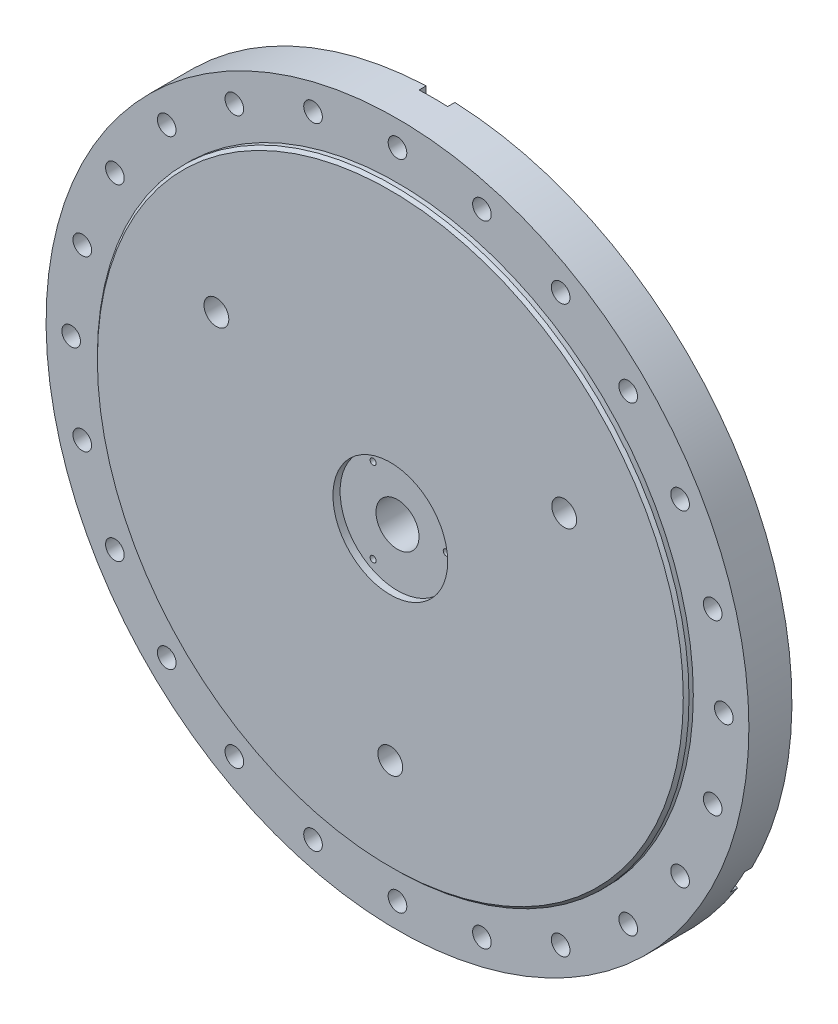
SolidWorks part; units mm, degrees
ref_plane "Front Plane" through (0, 0, 0) normal (0, 0, 1) x (1, 0, 0)
ref_plane "Top Plane" through (0, 0, 0) normal (0, 1, 0) x (1, 0, 0)
ref_plane "Right Plane" through (0, 0, 0) normal (1, 0, 0) x (0, 0, -1)
sketch "Sketch1" plane through (0, 0, 0) normal (0, 0, 1) x (1, 0, 0)
  circle A50 centre (114.9929, 70) radius 8.647 construction
  circle A51 centre (97.4929, 100.3109) radius 1.621 construction
  circle A52 centre (132.4929, 39.6891) radius 1.621 construction
  circle A53 centre (13.7494, 235) radius 2.067 construction
  circle A54 centre (207.2653, -100.1795) radius 2.067 construction
  circle A55 centre (214.9531, -72.8638) radius 2.4585 construction
  circle A56 centre (201.0967, -64.8638) radius 2.4585 construction
  circle A57 centre (187.2403, -56.8638) radius 2.4585 construction
  circle A58 centre (173.3839, -48.8638) radius 2.4585 construction
  circle A59 centre (159.5275, -40.8638) radius 2.4585 construction
  circle A60 centre (145.6711, -32.8638) radius 2.4585 construction
  circle A61 centre (131.8147, -24.8638) radius 2.4585 construction
  circle A62 centre (117.9583, -16.8638) radius 2.4585 construction
  circle A63 centre (104.1019, -8.8638) radius 2.4585 construction
  circle A64 centre (90.2455, -0.8638) radius 2.4585 construction
  circle A65 centre (76.3891, 7.1362) radius 2.4585 construction
  circle A66 centre (62.5327, 15.1362) radius 2.4585 construction
  circle A67 centre (48.6763, 23.1362) radius 2.4585 construction
  circle A68 centre (34.8199, 31.1362) radius 2.4585 construction
  circle A69 centre (41.2494, 228) radius 2.4585 construction
  circle A70 centre (41.2494, 212) radius 2.4585 construction
  circle A71 centre (41.2494, 196) radius 2.4585 construction
  circle A72 centre (41.2494, 180) radius 2.4585 construction
  circle A73 centre (41.2494, 164) radius 2.4585 construction
  circle A74 centre (41.2494, 148) radius 2.4585 construction
  circle A75 centre (41.2494, 132) radius 2.4585 construction
  circle A76 centre (41.2494, 116) radius 2.4585 construction
  circle A77 centre (41.2494, 100) radius 2.4585 construction
  circle A78 centre (41.2494, 84) radius 2.4585 construction
  circle A79 centre (41.2494, 68) radius 2.4585 construction
  circle A80 centre (41.2494, 52) radius 2.4585 construction
  circle A81 centre (41.2494, 36) radius 2.4585 construction
  circle A82 centre (41.2494, 20) radius 2.4585 construction
  circle A83 centre (-127.4942, 70) radius 8.647 construction
  circle A84 centre (-144.9942, 39.6891) radius 1.621 construction
  circle A85 centre (-109.9942, 100.3109) radius 1.621 construction
  circle A86 centre (-219.7666, -100.1795) radius 2.067 construction
  circle A87 centre (-26.2506, 235) radius 2.067 construction
  circle A88 centre (-227.4544, -72.8638) radius 2.4585 construction
  circle A89 centre (-213.598, -64.8638) radius 2.4585 construction
  circle A90 centre (-199.7416, -56.8638) radius 2.4585 construction
  circle A91 centre (-185.8852, -48.8638) radius 2.4585 construction
  circle A92 centre (-172.0288, -40.8638) radius 2.4585 construction
  circle A93 centre (-158.1724, -32.8638) radius 2.4585 construction
  circle A94 centre (-144.316, -24.8638) radius 2.4585 construction
  circle A95 centre (-130.4596, -16.8638) radius 2.4585 construction
  circle A96 centre (-116.6032, -8.8638) radius 2.4585 construction
  circle A97 centre (-102.7468, -0.8638) radius 2.4585 construction
  circle A98 centre (-88.8904, 7.1362) radius 2.4585 construction
  circle A99 centre (-75.034, 15.1362) radius 2.4585 construction
  circle A100 centre (-61.1776, 23.1362) radius 2.4585 construction
  circle A101 centre (-47.3212, 31.1362) radius 2.4585 construction
  circle A102 centre (-53.7506, 228) radius 2.4585 construction
  circle A103 centre (-53.7506, 212) radius 2.4585 construction
  circle A104 centre (-53.7506, 196) radius 2.4585 construction
  circle A105 centre (-53.7506, 180) radius 2.4585 construction
  circle A106 centre (-53.7506, 164) radius 2.4585 construction
  circle A107 centre (-53.7506, 148) radius 2.4585 construction
  circle A108 centre (-53.7506, 132) radius 2.4585 construction
  circle A109 centre (-53.7506, 116) radius 2.4585 construction
  circle A110 centre (-53.7506, 100) radius 2.4585 construction
  circle A111 centre (-53.7506, 84) radius 2.4585 construction
  circle A112 centre (-53.7506, 68) radius 2.4585 construction
  circle A113 centre (-53.7506, 52) radius 2.4585 construction
  circle A114 centre (-53.7506, 36) radius 2.4585 construction
  circle A115 centre (-53.7506, 20) radius 2.4585 construction
  circle A116 centre (-6.2506, -140) radius 8.647 construction
  circle A117 centre (28.7494, -140) radius 1.621 construction
  circle A118 centre (-41.2506, -140) radius 1.621 construction
  circle A119 centre (-199.7666, -134.8205) radius 2.067 construction
  circle A120 centre (187.2653, -134.8205) radius 2.067 construction
  circle A121 centre (167.4531, -155.1362) radius 2.4585 construction
  circle A122 centre (153.5967, -147.1362) radius 2.4585 construction
  circle A123 centre (139.7403, -139.1362) radius 2.4585 construction
  circle A124 centre (125.8839, -131.1362) radius 2.4585 construction
  circle A125 centre (112.0275, -123.1362) radius 2.4585 construction
  circle A126 centre (98.1711, -115.1362) radius 2.4585 construction
  circle A127 centre (84.3147, -107.1362) radius 2.4585 construction
  circle A128 centre (70.4583, -99.1362) radius 2.4585 construction
  circle A129 centre (56.6019, -91.1362) radius 2.4585 construction
  circle A130 centre (42.7455, -83.1362) radius 2.4585 construction
  circle A131 centre (28.8891, -75.1362) radius 2.4585 construction
  circle A132 centre (15.0327, -67.1362) radius 2.4585 construction
  circle A133 centre (1.1763, -59.1362) radius 2.4585 construction
  circle A134 centre (-179.9544, -155.1362) radius 2.4585 construction
  circle A135 centre (-166.098, -147.1362) radius 2.4585 construction
  circle A136 centre (-152.2416, -139.1362) radius 2.4585 construction
  circle A137 centre (-138.3852, -131.1362) radius 2.4585 construction
  circle A138 centre (-124.5288, -123.1362) radius 2.4585 construction
  circle A139 centre (-110.6724, -115.1362) radius 2.4585 construction
  circle A140 centre (-96.816, -107.1362) radius 2.4585 construction
  circle A141 centre (-82.9596, -99.1362) radius 2.4585 construction
  circle A142 centre (-69.1032, -91.1362) radius 2.4585 construction
  circle A143 centre (-55.2468, -83.1362) radius 2.4585 construction
  circle A144 centre (-41.3904, -75.1362) radius 2.4585 construction
  circle A145 centre (-27.534, -67.1362) radius 2.4585 construction
  circle A146 centre (-13.6776, -59.1362) radius 2.4585 construction
  circle A147 centre (-12.6801, -51.1362) radius 2.4585 construction
  circle A148 centre (0.1788, -51.1362) radius 2.4585 construction
  circle A149 centre (-6.2506, 0) radius 15 construction
  circle A150 centre (-233.7506, 0) radius 6.5 construction
  circle A151 centre (-167.1174, 160.8668) radius 6.5 construction
  circle A152 centre (-6.2506, 227.5) radius 6.5 construction
  circle A153 centre (52.6307, 219.7481) radius 6.5 construction
  circle A154 centre (-167.1174, -160.8668) radius 6.5 construction
  circle A155 centre (-203.2714, 113.75) radius 6.5 construction
  circle A156 centre (213.4975, -58.8813) radius 6.5 construction
  circle A157 centre (154.6161, 160.8668) radius 6.5 construction
  circle A158 centre (107.4994, 197.0208) radius 6.5 construction
  circle A159 centre (-225.9988, 58.8813) radius 6.5 construction
  circle A160 centre (-65.132, -219.7481) radius 6.5 construction
  circle A161 centre (154.6161, -160.8668) radius 6.5 construction
  circle A162 centre (-203.2714, -113.75) radius 6.5 construction
  circle A163 centre (190.7701, -113.75) radius 6.5 construction
  circle A164 centre (-6.2506, -227.5) radius 6.5 construction
  circle A165 centre (-225.9988, -58.8813) radius 6.5 construction
  circle A166 centre (-120.0006, -197.0208) radius 6.5 construction
  circle A167 centre (-120.0006, 197.0208) radius 6.5 construction
  circle A168 centre (-65.132, 219.7481) radius 6.5 construction
  circle A169 centre (221.2494, 0) radius 6.5 construction
  circle A170 centre (213.4975, 58.8813) radius 6.5 construction
  circle A171 centre (52.6307, -219.7481) radius 6.5 construction
  circle A172 centre (107.4994, -197.0208) radius 6.5 construction
  circle A173 centre (190.7701, 113.75) radius 6.5 construction
  circle A174 centre (-6.2506, 0) radius 245
extrude "Boss-Extrude2" add sketch "Sketch1" along normal blind 30
hole_wizard "Size mm Dowel hole 1" positions "Sketch3" profile "Sketch4" hole size "Ø5.0" standard "GB"
sketch "Sketch3" plane through (0, 0, 0) normal (0, 0, -1) x (-1, 0, 0)
  point P0 (-41.2494, 228)
  point P6 (-41.2494, 212)
  point P9 (-41.2494, 196)
  point P12 (-41.2494, 180)
  point P15 (-41.2494, 164)
  point P18 (-41.2494, 148)
  point P21 (-41.2494, 132)
  point P24 (-41.2494, 116)
  point P27 (-41.2494, 100)
  point P30 (-41.2494, 84)
  point P33 (-41.2494, 68)
  point P36 (-41.2494, 52)
  point P39 (-41.2494, 36)
  point P42 (-34.8199, 31.1362)
sketch "Sketch4" plane through (41.2494, 228, 0) normal (1, 0, 0) x (0, 1, 0)
  line L0 (0, 0) -> (0, 18.6022)
  line L1 (0, 18.6022) -> (2.5, 17.1)
  line L2 (2.5, 17.1) -> (2.5, 0)
  line L5 (2.5, 0) -> (0, 0)
  line L10 (0, 18.6022) -> (-2.5, 17.1) construction
  line L11 (0, -6.35) -> (0, 107.95) construction
  dimension "孔直径" = 5
  dimension "孔深度" = 17.1
  dimension "导头角度" = 118
sketch "Sketch5" plane through (0, 0, 0) normal (0, 0, -1) x (-1, 0, 0)
  line L0 (6.2506, 0) -> (6.2506, 73.1913) construction
ref_plane "Plane3" through (-6.2506, 0, 0) normal (-1, 0, 0) x (0, 1, 0)
mirror "Mirror2" about plane through (-6.2506, 0, 0) normal (-1, 0, 0) of "Size mm Dowel hole 1"
pattern_circular "CirPattern2" count 3 over 360 about axis through (-6.2506, 0, 0) along (0, 0, 1) of "Mirror2", "Size mm Dowel hole 1"
sketch "Sketch6" plane through (0, 0, 0) normal (0, 0, -1) x (-1, 0, 0)
  line L0 (-3.7494, -45) -> (16.2506, -45)
  line L1 (16.2506, 297.9704) -> (-3.7494, 297.9704)
  line L2 (16.2506, 297.9704) -> (16.2506, 17.3205)
  line L4 (-3.7494, 297.9704) -> (-3.7494, 17.3205)
  line L5 (16.2506, 297.9704) -> (-3.7494, 6.6139) construction
  line L6 (16.2506, 6.6139) -> (-3.7494, 297.9704) construction
  line L7 (6.2506, -20) -> (33.6197, -20) construction
  line L8 (-3.7494, -17.3205) -> (-3.7494, -45)
  line L9 (16.2506, -17.3205) -> (16.2506, -45)
  arc A0 (-3.7494, 17.3205) -> (-3.7494, -17.3205) centre (6.2506, 0) ccw
  arc A1 (16.2506, -17.3205) -> (16.2506, 17.3205) centre (6.2506, 0) ccw
  point P3 (6.2506, 152.2921)
  dimension "D1" = 40
  dimension "D2" = 20
  dimension "D3" = 25
hole_wizard "Size mm Dowel hole 4" positions "Sketch17" profile "Sketch18" hole size "Ø5.0" standard "GB"
sketch "Sketch17" plane through (0, 0, 0) normal (0, 0, -1) x (-1, 0, 0)
  point P0 (-13.7494, 235)
  point P3 (26.2506, 235)
  point P6 (219.7666, -100.1795)
  point P9 (199.7666, -134.8205)
  point P12 (-207.2653, -100.1795)
  point P15 (-187.2653, -134.8205)
sketch "Sketch18" plane through (13.7494, 235, 0) normal (1, 0, 0) x (0, 1, 0)
  line L0 (0, 0) -> (0, 15.4618)
  line L1 (0, 15.4618) -> (2.1, 14.2)
  line L2 (2.1, 14.2) -> (2.1, 0)
  line L5 (2.1, 0) -> (0, 0)
  line L10 (0, 15.4618) -> (-2.1, 14.2) construction
  line L11 (0, -6.35) -> (0, 107.95) construction
  dimension "孔直径" = 4.2
  dimension "孔深度" = 14.2
  dimension "导头角度" = 118
extrude "Cut-Extrude1" cut sketch "Sketch6" against normal blind 5
pattern_circular "CirPattern3" count 3 over 360 about axis through (-6.2506, 0, 0) along (0, 0, 1) of "Cut-Extrude1"
sketch "Sketch7" plane through (0, 0, 5) normal (0, 0, -1) x (-1, 0, 0)
  circle A1 centre (6.2506, 0) radius 15
  dimension "D1" = 30
extrude "Cut-Extrude2" cut sketch "Sketch7" against normal through all
hole_wizard "大小mm 暗销孔4" positions "Sketch8" profile "Sketch9" hole size "Ø3.0" standard "GB"
sketch "Sketch8" plane through (0, 0, 0) normal (0, 0, -1) x (-1, 0, 0)
  point P0 (-97.4929, 100.3109)
  point P3 (-132.4929, 39.6891)
  point P6 (109.9942, 100.3109)
  point P9 (144.9942, 39.6891)
  point P12 (41.2506, -140)
  point P15 (-28.7494, -140)
sketch "Sketch9" plane through (97.4929, 100.3109, 0) normal (1, 0, 0) x (0, 1, 0)
  line L0 (0, 0) -> (0, 12.7614)
  line L1 (0, 12.7614) -> (1.6, 11.8)
  line L2 (1.6, 11.8) -> (1.6, 0)
  line L5 (1.6, 0) -> (0, 0)
  line L10 (0, 12.7614) -> (-1.6, 11.8) construction
  line L11 (0, -6.35) -> (0, 107.95) construction
  dimension "孔直径" = 3.2
  dimension "孔深度" = 11.8
  dimension "导头角度" = 118
sketch "Sketch10" plane through (0, 0, 0) normal (0, 0, -1) x (-1, 0, 0)
  circle A0 centre (-114.9929, 70) radius 8.647
  circle A1 centre (127.4942, 70) radius 8.647
  circle A2 centre (6.2506, -140) radius 8.647
  circle A3 centre (-190.7701, 113.75) radius 6.5
  circle A27 centre (-154.6161, 160.8668) radius 6.5
  circle A28 centre (-107.4994, 197.0208) radius 6.5
  circle A29 centre (-52.6307, 219.7481) radius 6.5
  circle A30 centre (6.2506, 227.5) radius 6.5
  circle A31 centre (65.132, 219.7481) radius 6.5
  circle A32 centre (120.0006, 197.0208) radius 6.5
  circle A33 centre (167.1174, 160.8668) radius 6.5
  circle A34 centre (203.2714, 113.75) radius 6.5
  circle A35 centre (225.9988, 58.8813) radius 6.5
  circle A36 centre (233.7506, 0) radius 6.5
  circle A37 centre (225.9988, -58.8813) radius 6.5
  circle A38 centre (203.2714, -113.75) radius 6.5
  circle A39 centre (167.1174, -160.8668) radius 6.5
  circle A40 centre (120.0006, -197.0208) radius 6.5
  circle A41 centre (65.132, -219.7481) radius 6.5
  circle A42 centre (6.2506, -227.5) radius 6.5
  circle A43 centre (-52.6307, -219.7481) radius 6.5
  circle A44 centre (-107.4994, -197.0208) radius 6.5
  circle A45 centre (-154.6161, -160.8668) radius 6.5
  circle A46 centre (-190.7701, -113.75) radius 6.5
  circle A47 centre (-213.4975, -58.8813) radius 6.5
  circle A48 centre (-221.2494, 0) radius 6.5
  circle A49 centre (-213.4975, 58.8813) radius 6.5
  point P61 (6.2506, 0)
extrude "Cut-Extrude3" cut sketch "Sketch10" against normal through all
sketch "Sketch12" plane through (0, 0, 0) normal (0, 0, -1) x (-1, 0, 0)
  circle A0 centre (-154.6161, 160.8668) radius 10
  circle A24 centre (-107.4994, 197.0208) radius 10
  circle A25 centre (-52.6307, 219.7481) radius 10
  circle A26 centre (6.2506, 227.5) radius 10
  circle A27 centre (65.132, 219.7481) radius 10
  circle A28 centre (120.0006, 197.0208) radius 10
  circle A29 centre (167.1174, 160.8668) radius 10
  circle A30 centre (203.2714, 113.75) radius 10
  circle A31 centre (225.9988, 58.8813) radius 10
  circle A32 centre (233.7506, 0) radius 10
  circle A33 centre (225.9988, -58.8813) radius 10
  circle A34 centre (203.2714, -113.75) radius 10
  circle A35 centre (167.1174, -160.8668) radius 10
  circle A36 centre (120.0006, -197.0208) radius 10
  circle A37 centre (65.132, -219.7481) radius 10
  circle A38 centre (6.2506, -227.5) radius 10
  circle A39 centre (-52.6307, -219.7481) radius 10
  circle A40 centre (-107.4994, -197.0208) radius 10
  circle A41 centre (-154.6161, -160.8668) radius 10
  circle A42 centre (-190.7701, -113.75) radius 10
  circle A43 centre (-213.4975, -58.8813) radius 10
  circle A44 centre (-221.2494, 0) radius 10
  circle A45 centre (-213.4975, 58.8813) radius 10
  circle A46 centre (-190.7701, 113.75) radius 10
  point P52 (6.2506, 0)
extrude "Cut-Extrude4" cut sketch "Sketch12" against normal blind 20
sketch "Sketch13" plane through (0, 0, 30) normal (0, 0, 1) x (1, 0, 0)
  circle A0 centre (-6.2506, 0) radius 206.25
  circle A1 centre (-6.2506, 0) radius 40
  circle A2 centre (-127.4942, 70) radius 8.647
  circle A3 centre (114.9929, 70) radius 8.647
  circle A4 centre (-6.2506, -140) radius 8.647
  dimension "D1" = 412.5
  dimension "D2" = 80
extrude "Boss-Extrude3" add sketch "Sketch13" along normal blind 5
sketch "Sketch14" plane through (0, 0, 30) normal (0, 0, 1) x (1, 0, 0)
  circle A0 centre (-6.2506, 0) radius 34 construction
  circle A1 centre (27.7494, 0) radius 7.8114
  circle A2 centre (-23.2506, -29.4449) radius 7.8114
  circle A3 centre (-23.2506, 29.4449) radius 7.8114
  point P12 (-6.2506, 0)
  dimension "D1" = 68
  dimension "D2" = 3
hole_wizard "大小mm 暗销孔4" positions "Sketch15" profile "Sketch16" hole size "Ø4.0" standard "GB"
sketch "Sketch15" plane through (0, 0, 35) normal (0, 0, 1) x (1, 0, 0)
  point P0 (-23.2506, 29.4449)
  point P3 (-23.2506, -29.4449)
  point P6 (27.7494, 0)
sketch "Sketch16" plane through (-23.2506, 29.4449, 35) normal (1, 0, 0) x (0, -1, 0)
  line L0 (0, 0) -> (0, 15.4618)
  line L1 (0, 15.4618) -> (2.1, 14.2)
  line L2 (2.1, 14.2) -> (2.1, 0)
  line L5 (2.1, 0) -> (0, 0)
  line L10 (0, 15.4618) -> (-2.1, 14.2) construction
  line L11 (0, -6.35) -> (0, 107.95) construction
  dimension "孔直径" = 4.2
  dimension "孔深度" = 14.2
  dimension "导头角度" = 118
chamfer "Chamfer1" distance 2 angle 45 1 edges at (199.9994, 0, 35)
